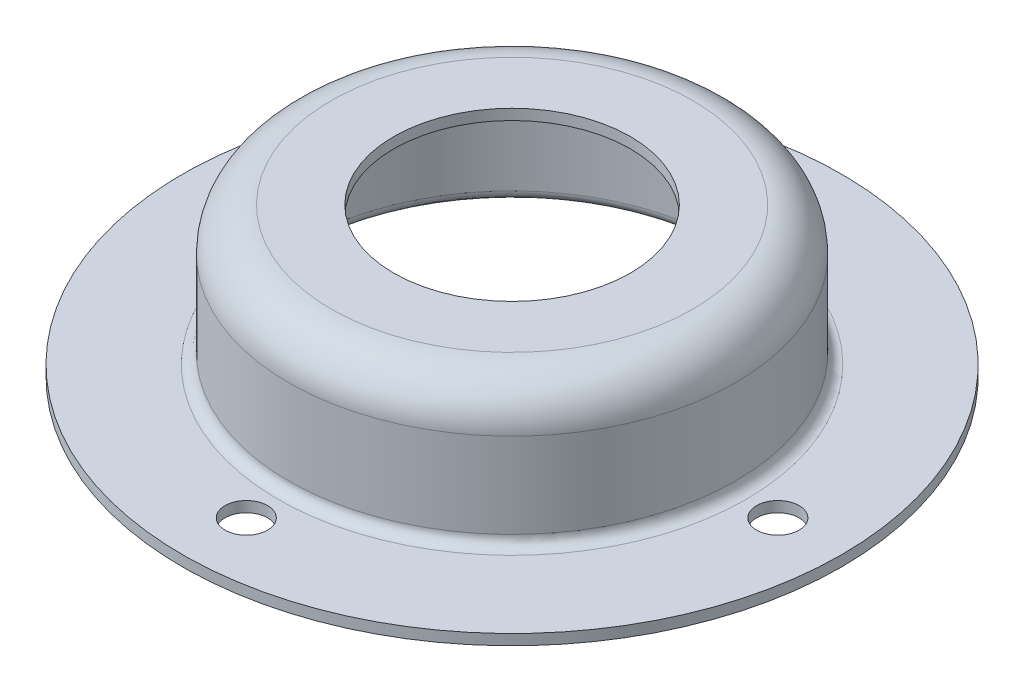
SolidWorks part; units mm, degrees
ref_plane "前视基准面" through (0, 0, 0) normal (0, 0, 1) x (1, 0, 0)
ref_plane "上视基准面" through (0, 0, 0) normal (0, 1, 0) x (1, 0, 0)
ref_plane "右视基准面" through (0, 0, 0) normal (1, 0, 0) x (0, 0, -1)
sketch "草图1" plane through (0, 0, 0) normal (0, 0, 1) x (1, 0, 0)
  line L0 (0, 13) -> (0, 12)
  line L2 (0, 13) -> (17, 13)
  line L3 (21, 9) -> (21, 1)
  line L4 (22, 0) -> (31, 0)
  line L7 (0, 12) -> (16, 12)
  line L8 (20, 8) -> (20, 0)
  line L9 (21, -1) -> (31, -1)
  line L11 (31, 0) -> (31, -1)
  line L12 (20, 12) -> (20, -1) construction
  line L13 (20, -1) -> (31, -1) construction
  line L14 (21, 13) -> (21, 0) construction
  line L15 (21, 0) -> (31, 0) construction
  line L16 (-32, -1) -> (-21, -1) construction
  line L17 (-21, -1) -> (-21, 12) construction
  line L18 (-32, 0) -> (-22, 0) construction
  line L19 (-22, 0) -> (-22, 13) construction
  line L20 (-22, 13) -> (21, 13) construction
  line L21 (-21, 12) -> (20, 12) construction
  line L22 (0, 0) -> (0, 13) construction
  arc A0 (20, 0) -> (21, -1) centre (21, 0) ccw
  arc A1 (21, 1) -> (22, 0) centre (22, 1) ccw
  arc A6 (20, 8) -> (16, 12) centre (16, 8) ccw
  arc A7 (21, 9) -> (17, 13) centre (17, 9) ccw
  point P19 (21, 0)
  point P26 (-22, 0)
  dimension "D6" = 1
  dimension "D1" = 4
  dimension "D2" = 12
  dimension "D3" = 10
  dimension "D4" = 20
  dimension "D5" = 1
revolve "旋转3" add sketch "草图1" angle 360 about L22
sketch "草图2" plane through (0, 0, 0) normal (0, 1, 0) x (1, 0, 0)
  circle A0 centre (0, 0) radius 25 construction
  circle A1 centre (0, 25) radius 2
  circle A2 centre (25, 0) radius 2
  circle A3 centre (0, -25) radius 2
  circle A4 centre (-25, 0) radius 2
  dimension "D1" = 50
  dimension "D2" = 4
extrude "切除-拉伸1" cut sketch "草图2" against normal up to surface (1 mm away) up to face at (31, -1, 0)
sketch "草图3" plane through (0, 13, 0) normal (0, 1, 0) x (1, 0, 0)
  circle A0 centre (0, 0) radius 11.13
  dimension "D1" = 22.26
extrude "切除-拉伸2" cut sketch "草图3" against normal blind 10
